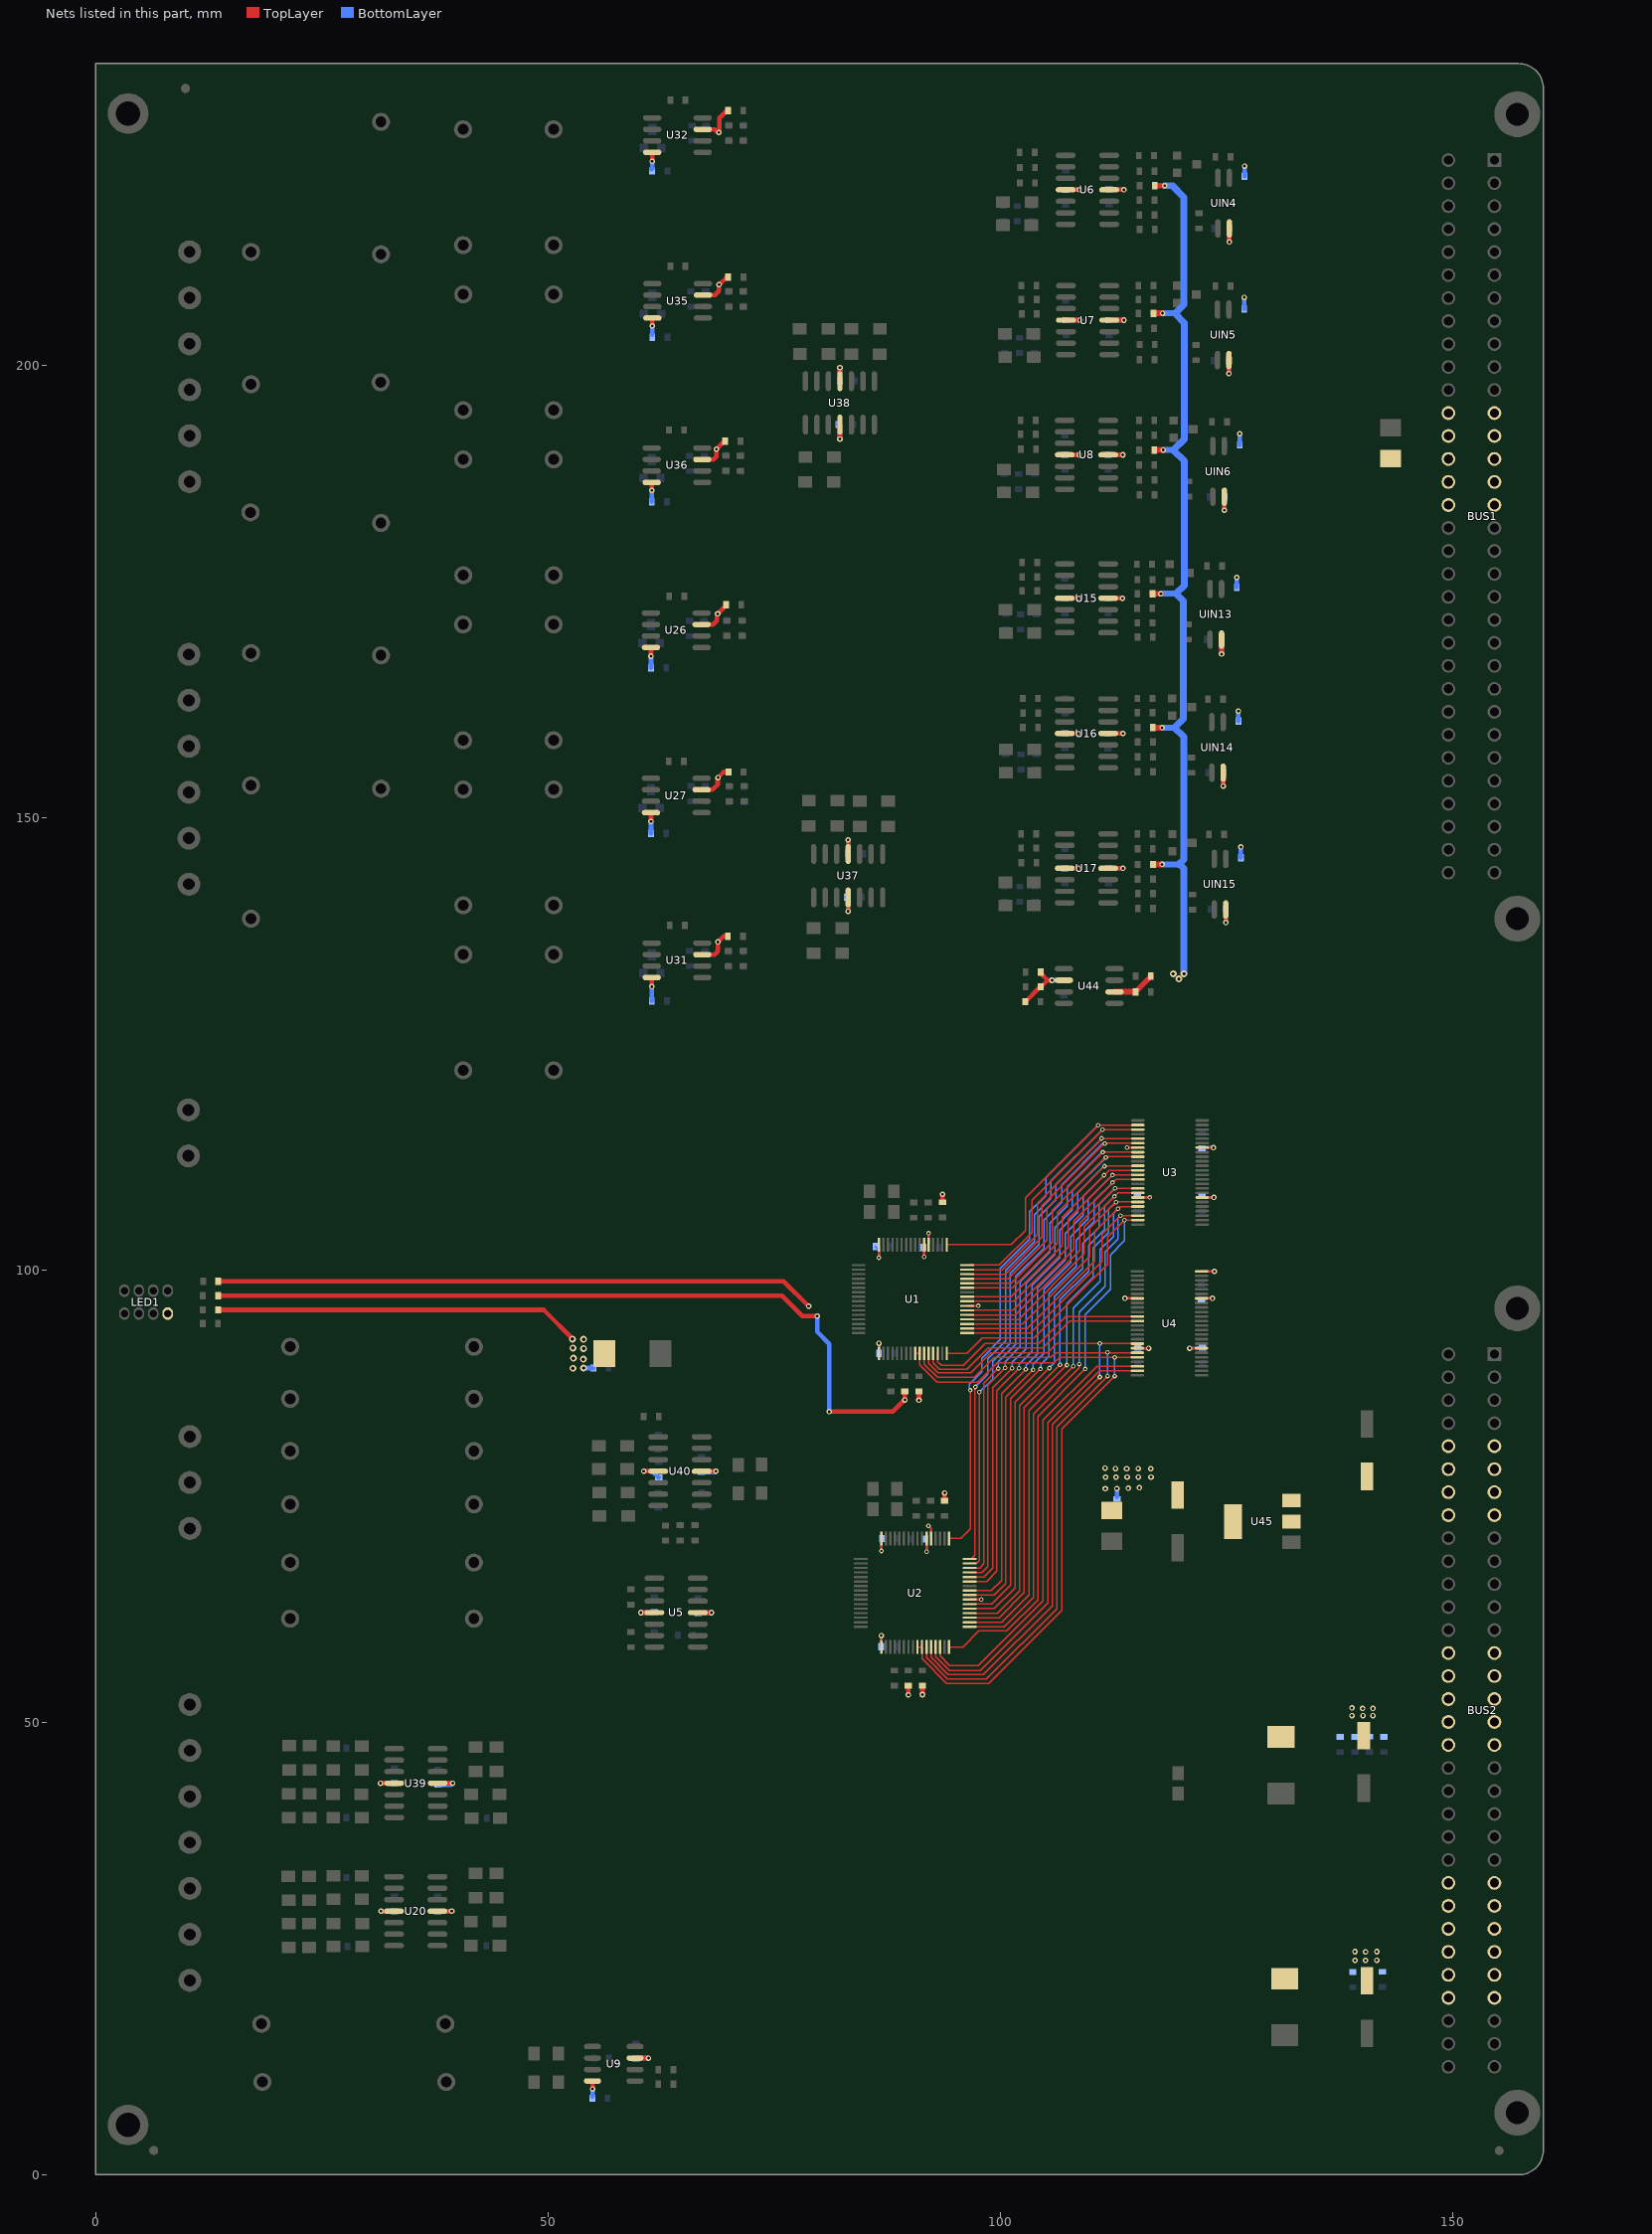
[diagram p0: the nets of this part, all layers, seen from the top]
# Altium PCB MISC80584.PCBDoc (part 3 of 7)
Units mm, origin at the board's own origin, x right, y up, seen from the top; angles counter-clockwise.
Board outline 160.02 x 233.3 mm, 4 copper layers (TopLayer, GND, POWER, BottomLayer); 386 components, 266 nets, 1374 pads, 640 vias.

## Part data
BUS1 BUS2: "Euro-style pin header, 64 positions"
C1 C2 C3 C7 C8 C18 C19 C22 C24 C25 C26 C119 C120 C121 C122 C123 C124 C128 C129 C156 C157 C158 C159 C163 C164 C165 C171 C173 C174 C175 C176 C177 C178 C179 C180 C181 C182 C183 C184 C192 C193 C194 C195 C196 C197 C204 C205 C206 C215 C216 C217 C218 C219 C220 C224 C230 C231 C232 C233 C234 C235 C238 C239 C240 C249 C251 C252 C253 C254 C255 C256 C257 C261 C262: library part CAP, "Capacitor"
C4 C5 C6 C9 C10 C11 C12 C13 C14 C15 C16 C17 C20 C21 C23 C27 C82 C83 C84 C85 C88 C89 C92 C93 C96 C97 C100 C101 C104 C113 C118 C125 C126 C130 C132 C135 C136 C139 C142 C143 C146 C147 C148 C149: library part CAP
CT1 CT2 CT3 CT17: library part EC
CT4 CT7 CT8 CT13 CT16: library part "CAPACITOR POL", "Capacitor"
D1 D2 D8 D9 D10 D11 D12 D13 D14 D15 D16 D17 D18 D20 D21 D22 D24 D25 D26 D27 D28 D29 D30 D31 D32 D33 D60 D61 D62 D63 D64 D65 D80 D81 D83 D84 D85 D89 D90 D91 D94 D95 D96 D97: library part DIODE-S
D42 D44 D46 D48 D51 D53: library part DDIODEB
J1 J2: "Connector"
L1: library part INDUCTOR
Q8 Q9 Q10 Q17 Q23 Q24: library part NPN, "NPN Transistor"
R1 R2 R3 R4 R5 R6 R7 R8 R9 R10 R11 R12 R13 R14 R23 R24 R25 R26 R27 R28 R29 R30 R31 R32 R33 R34 R35 R36 R37 R38 R40 R48 R57 R58 R59 R67 R70 R71 R76 R85 R86 R87 R93 R97 R100 R105 R106 R108 R110 R111 R113 R117 R118 R119 R120 R124 R125 R126 R130 R131 R132 R133 R137 R138 R139 R145 R146 R147 R150 R151 R152 R155 R156 R157 R161 R162 R165 R168 R171 R174 R211 R224 R225 R339 R340 R341 R342 R349 R350 R351 R353 R354 R355 R357 R358 R359 R360 R361 R362 R364 R365 R366 R372 R373 R374 R375 R376 R377 R379 R380 R381 R382 R383 R384 R399 R400 R401 R414 R423 R430 R431 R435 R437 R438 R444 R445 R446 R450 R451 R452 R459 R460 R461 R486 R487 R488 R491 R492 R493 R503 R506 R507 R510 R511 R512 R591 R592 R593 R600 R601 R602 R605 R607 R608 R609 R611 R612: library part RES2
SPT1 SPT2 SPT3 SPT4 SPT5 SPT6: library part SPT
U3 U4: library part SN74LVCH16T245, "TI SN74LVCH16T245DGGR"
U5 U20 U37 U38 U39 U40: "Low Power Quad Operational Amplifier"
U6 U7 U8 U15 U16 U17: library part TL084
U26 U27 U31 U32 U35 U36: library part LM101
U44: "U?"
U45: library part 7810
UIN4 UIN5 UIN6 UIN13 UIN14 UIN15: library part 521-1, "Optoisolator"

## Free pads (board coordinates)
  round 1 smd mask+1.5: 0(6.426,2.718) 0(9.931,230.581) 0(155.143,2.692)
  round 1 smd far side mask+1.5: 0(6.426,2.718) 0(9.931,230.581) 0(155.143,2.692)
  round 4.5 hole 2.7: 1(3.592,5.524) 1(3.592,227.823)

## Via types
v1: diameter 0.61, hole 0.305, TopLayer to BottomLayer, 342 vias
v2: diameter 0.762, hole 0.381, TopLayer to BottomLayer, 197 vias
v3: diameter 0.508, hole 0.254, TopLayer to BottomLayer, 101 vias

## Nets (pads, with @x,y where several pads share a name; then routed paths per layer and width w, separated by ;. In a path a pad name is that pad's centre, name@x,y a point inside that pad or via, vN(x,y) a via of type N, cw(c..) or ccw(c..) an arc to the next point about the centre after c; other vN are vias at no path point)
+3.3V: C1.2 C3.1 C8.1 CT16.1 CT17.1 R33.2 R34.2 R342.2 R605.2 R607.2 R609.2 R611.2 U1.23 U2.23 U3.7 U3.18 U4.24 U4.31 U4.42 U45.2 | length 105.4
  TopLayer w0.254: U1.23@96.339,96.055 v3(97.579,96.055) ; U2.23@96.593,63.594 v3(97.884,63.594)
  TopLayer w0.279: v1(113.764,96.873) U4.31@115.15,96.873 ; v3(113.979,113.529) U3.7@115.214,113.529 ; U4.42@115.15,91.373 v1(116.392,91.373) ; U3.18@115.214,108.029 v3(116.507,108.029) ; U4.24@122.25,99.873 v1(123.673,99.873)
  TopLayer w0.508: R342.2@13.538,97.18 75.87,97.18 78.13,94.92 v1(79.756,94.92) ; v1(81.102,84.353) 88.113,84.353 v1@89.408,85.649 ; v1(89.459,85.649) R607.2@89.459,86.589 ; v1(89.84,53.061) R611.2@89.84,54.077 ; v1(91.008,85.623) R605.2@91.008,86.589 ; v1(91.389,53.086) R609.2@91.389,54.077 ; R33.2@93.624,107.493 v1(93.624,108.382) ; R34.2@93.853,74.524 v1(93.853,75.387)
  BottomLayer w0.254: v3(97.579,96.055) v3@97.612,96.088 ; v3(97.884,63.594) v3@97.892,63.602
  BottomLayer w0.279: v1@113.741,96.85 v1(113.764,96.873) ; C8.1@115.138,108.052 116.357,108.052 v3@116.408,108.001 ; C1.2@115.189,91.364 v1@116.256,91.364 ; v1(116.392,91.373) v1@116.484,91.465 ; v3(116.507,108.029) v3@116.51,108.026
  BottomLayer w0.508: v1(79.756,94.92) 79.756,93.193 81.102,91.846 v1(81.102,84.353) ; v1@89.433,85.623 v1(89.459,85.649) ; v1@112.878,75.819 112.878,74.981 C3.1@112.903,74.955
  other v1: 111.608,75.844 112.878,75.87 114.148,75.895 115.367,75.946 111.633,77.114 112.776,77.114 114.021,77.14 115.265,77.14 116.662,77.14 113.97,78.054 116.637,78.054 112.725,78.08 115.24,78.08 111.582,78.13
+5V: BUS1.A12 BUS1.A13 BUS1.A14 BUS1.A15 BUS1.A16 BUS1.C12 BUS1.C13 BUS1.C14 BUS1.C15 BUS1.C16 BUS2.A5 BUS2.A6 BUS2.A7 BUS2.A8 BUS2.C5 BUS2.C6 BUS2.C7 BUS2.C8 C2.1 C7.2 C18.1 C24.1 C119.1 C120.1 C128.1 C129.1 C156.2 C157.1 C158.1 C159.2 C163.1 C164.1 C165.2 C171.1 CT1.1 CT8.1 R339.2 U1.1 U1.37 U1.38 U1.48 U2.1 U2.37 U2.38 U2.48 U3.31 U3.42 U4.7 U4.18 U45.3 UIN4.4 UIN5.4 UIN6.4 UIN13.4 UIN14.4 UIN15.4 | length 111.3
  TopLayer w0.254: v3(86.589,101.371) U1.48@86.589,102.805 ; U2.1@86.843,58.344 v1(86.843,59.614) ; v3(86.843,68.961) U2.48@86.843,70.344 ; v3(91.589,101.444) U1.38@91.589,102.805 ; v3(91.843,68.889) U2.38@91.843,70.344 ; v3(92.05,71.73) 92.343,71.437 U2.37@92.343,70.344 ; v3(92.061,104.076) 92.089,104.076 U1.37@92.089,102.805
  TopLayer w0.279: U1.1@86.589,90.805 v1@86.589,91.948 ; v1(120.938,91.373) U4.7@122.25,91.373 ; U4.18@122.25,96.873 v1(123.441,96.873) ; U3.31@122.314,108.029 v1(123.619,108.029) ; U3.42@122.314,113.529 v1(123.562,113.529)
  TopLayer w0.508: R339.2@13.564,98.755 76.048,98.755 78.816,95.987 v1(78.816,96.012) ; v1(124.46,168.072) UIN13.4@124.46,169.672 ; v1(124.638,153.492) UIN14.4@124.638,154.965 ; v1(124.765,183.972) UIN6.4@124.765,185.471 ; v1(124.917,138.405) UIN15.4@124.917,139.852 ; v1(125.273,199.085) UIN5.4@125.273,200.558 ; v1(125.324,213.614) UIN4.4@125.324,215.113
  BottomLayer w0.254: C119.1@86.208,102.591 86.589,102.21 v3@86.589,101.448 ; C129.1@86.843,58.369 v1@86.843,59.436 ; v3@86.843,69.139 C24.1@86.843,70.333 ; C18.1@91.491,102.489 91.592,102.387 v3@91.592,101.524 ; v3@91.846,69.012 C120.1@91.846,70.358
  BottomLayer w0.279: C128.1@86.589,90.78 v1@86.589,91.821 ; v1@121.031,91.389 C2.1@122.326,91.389 ; C171.1@122.25,96.876 v1@123.317,96.876 ; C165.2@122.276,113.589 v1@123.52,113.589 ; C7.2@122.482,108.029 v1(123.619,108.029) ; v1(123.441,96.873) v1@123.444,96.876 ; v1(123.562,113.529) v1@123.571,113.538
  BottomLayer w0.508: v1(124.46,168.072) C159.2@124.46,169.469 ; v1(124.638,153.492) C163.1@124.638,154.813 ; v1(124.765,183.972) C158.1@124.765,185.268 ; C164.1@124.892,139.878 124.917,139.852 v1(124.917,138.405) ; v1(125.273,199.085) C157.1@125.273,200.457 ; v1(125.324,213.614) 125.324,214.96 C156.2@125.349,214.986
  other v1: 86.589,91.923
+5VREF: C148.1 C149.2 R155.2 R156.2 R157.2 R379.2 R380.2 R381.2 U44.6 | length 110.3
  TopLayer w0.635: U44.6@112.624,130.759 114.859,130.759 114.91,130.708 116.611,132.41 C149.2@116.611,132.486 ; R379.2@116.815,174.727 v1(117.754,174.727) ; R380.2@116.84,159.944 v1(117.881,159.944) ; R381.2@116.865,144.831 v1(117.881,144.831) ; R156.2@116.942,205.74 v1(117.932,205.74) ; R157.2@117.018,190.627 v1(118.008,190.627) ; R155.2@117.069,219.837 v1(118.161,219.837)
  BottomLayer w0.635: v1@117.78,174.752 119.405,174.752 ; v1@117.932,159.944 119.253,159.944 ; v1@117.983,144.831 119.71,144.831 ; v1@118.008,205.74 119.278,205.74 ; v1@118.034,190.627 119.151,190.627
  BottomLayer w0.762: v1(118.161,219.837) 119.024,219.837 120.294,218.567 120.294,206.705 119.329,205.74 119.278,205.74 120.345,204.673 120.345,191.821 119.151,190.627 119.126,190.602 119.151,190.602 120.345,189.408 120.345,175.666 119.431,174.752 120.218,173.965 120.218,160.909 119.253,159.944 120.269,158.928 120.269,145.39 119.71,144.831 119.837,144.831 120.269,144.399 v2@120.269,132.817
  other v2: 119.736,132.182 119.126,132.74 120.294,132.74
+15V: BUS2.A14 BUS2.A15 BUS2.A16 BUS2.A17 BUS2.A18 BUS2.C14 BUS2.C15 BUS2.C16 BUS2.C17 BUS2.C18 C146.1 C147.1 C173.2 C174.1 C175.1 C176.2 C177.1 C178.2 C179.2 C180.1 C181.1 C182.2 C183.2 C184.1 C215.1 C216.2 C217.2 C218.1 C219.2 C220.2 C224.1 C230.2 C231.1 C232.1 C233.2 C234.1 C235.2 CT2.1 CT4.1 CT7.1 R224.2 R340.2 R486.1 R487.1 R488.1 R503.1 R506.1 R507.1 U5.4 U6.4 U7.4 U8.4 U9.7 U15.4 U16.4 U17.4 U20.4 U26.7 U27.7 U31.7 U32.7 U35.7 U36.7 U37.4 U38.4 U39.4 U40.4 U44.2 | length 117.5
  TopLayer w0.508: R340.2@13.538,95.606 49.53,95.606 v2@52.73,92.405 ; v1(31.496,43.307) U39.4@33.008,43.307 ; v1(31.547,29.159) U20.4@32.982,29.159 ; U9.7@59.627,12.929 v1(61.112,12.929) ; v1(60.274,62.154) U5.4@61.76,62.154 ; v1(60.579,77.775) U40.4@62.192,77.775 ; U27.7@66.98,153.086 68.199,153.086 68.758,153.645 v1@68.758,154.381 ; U26.7@66.98,171.348 68.25,171.348 68.682,171.78 v1@68.682,172.441 ; U31.7@67.056,134.874 68.428,134.874 68.783,135.23 v1@68.783,136.246 ; U36.7@67.056,189.586 68.301,189.586 68.605,189.89 68.605,190.729 v1(68.631,190.729) C181.1@69.596,191.694 ; U32.7@67.107,226.06 68.453,226.06 v1@68.783,225.73 ; U35.7@67.132,207.747 68.478,207.747 68.91,208.178 v1@68.91,208.864 ; v1(68.758,172.517) v1@68.682,172.441 ; v1(68.783,136.271) v1@68.783,136.246 ; v1@68.796,225.742 v1@68.809,225.73 ; v1(68.809,154.432) v1@68.758,154.381 ; v1@68.809,225.704 v1@68.809,225.73 ; v1@68.834,225.704 v1@68.809,225.73 ; v1@68.834,225.781 v1@68.885,225.831 ; v1(68.885,225.704) v1@68.885,225.831 ; v1(68.91,208.915) v1@68.91,208.864 ; C180.1@69.672,173.431 v1@68.682,172.441 ; C184.1@69.748,209.702 v1@68.91,208.864 ; C183.2@69.774,228.143 68.961,227.33 68.961,225.908 v1@68.885,225.831 ; C178.2@69.85,136.881 69.418,136.881 v1@68.783,136.246 ; C179.2@69.952,155.042 69.418,155.042 v1@68.758,154.381 ; U38.4@82.271,198.234 v1(82.271,199.72) ; U37.4@83.185,145.986 v1(83.185,147.549) ; R224.2@102.768,129.667 C147.1@104.318,131.216 ; C147.1@104.572,131.369 105.232,132.029 ; C146.1@104.623,132.639 105.232,132.029 ; v1(105.715,132.029) 105.232,132.029 ; U17.4@107.125,144.399 v1(108.61,144.399) ; U16.4@107.125,159.309 v1(108.61,159.309) ; U15.4@107.125,174.244 v1(108.661,174.244) ; U8.4@107.125,190.094 v1(108.737,190.094) ; U6.4@107.226,219.38 v1(108.737,219.38) ; U7.4@107.252,204.978 v1(108.814,204.978)
  BottomLayer w0.508: v1(31.496,43.307) C235.2@32.817,43.307 ; v1@31.623,29.185 31.674,29.134 C230.2@33.045,29.134 ; v2@54.178,89.205 54.204,89.179 C182.2@55.016,89.179 ; C220.2@59.792,12.903 59.817,12.929 v1(61.112,12.929) ; v1(60.274,62.154) C177.1@61.62,62.154 ; v1@60.63,77.775 61.544,77.775 C234.1@62.23,77.089 ; v1(68.783,136.271) v1@68.809,136.296 ; C224.1@82.194,198.247 82.271,198.323 v1(82.271,199.72) ; C233.2@83.185,146.228 v1(83.185,147.549) ; v1(105.715,132.029) C216.2@106.909,132.029 ; C217.2@107.239,159.334 107.264,159.309 v1(108.61,159.309) ; C218.1@107.239,174.269 107.264,174.244 v1(108.661,174.244) ; C231.1@107.29,144.399 v1(108.61,144.399) ; C232.1@107.29,190.094 v1(108.737,190.094) ; C215.1@107.34,219.405 107.366,219.38 v1(108.737,219.38) ; C219.2@107.467,204.978 v1(108.814,204.978) ; R503.1@126.136,175.438 v1(126.136,176.555) ; R506.1@126.314,160.655 v1(126.314,161.773) ; R488.1@126.467,191.186 v1(126.467,192.43) ; R507.1@126.594,145.567 v1(126.594,146.761) ; R487.1@126.949,206.223 v1(126.949,207.493) ; R486.1@127,220.878 v1(127,221.996)
  other v1: 138.862,50.775 140.081,50.775 141.199,50.775 140.056,51.562 141.199,51.562 138.862,51.613
  other v2: 52.756,89.154 53.95,89.179 53.924,90.145 52.807,90.272 53.95,91.338 52.756,91.389 53.95,92.354 52.705,92.38
-15V: BUS2.A24 BUS2.A25 BUS2.A26 BUS2.A27 BUS2.A28 BUS2.A29 BUS2.C24 BUS2.C25 BUS2.C26 BUS2.C27 BUS2.C28 BUS2.C29 C192.2 C193.1 C194.2 C195.1 C196.1 C197.2 C204.2 C205.2 C206.1 C238.2 C239.1 C240.1 C249.1 C251.2 C252.1 C253.2 C254.1 C255.1 C256.2 C257.2 C261.2 C262.1 CT3.2 CT13.2 LED1.8 U5.11 U6.11 U7.11 U8.11 U9.4 U15.11 U16.11 U17.11 U20.11 U26.4 U27.4 U31.4 U32.4 U35.4 U36.4 U37.11 U38.11 U39.11 U40.11 | length 52.4
  TopLayer w0.508: U20.11@37.782,29.159 v1(39.37,29.159) ; U39.11@37.808,43.307 v1(39.472,43.307) ; v1(54.927,9.513) U9.4@54.927,10.389 ; v1(61.392,149.581) U27.4@61.392,150.546 ; v1(61.392,167.843) U26.4@61.392,168.808 ; v1(61.468,131.318) U31.4@61.468,132.334 ; v1(61.468,186.157) U36.4@61.468,187.046 ; v1(61.519,222.529) U32.4@61.519,223.52 ; v1(61.544,204.343) U35.4@61.544,205.207 ; U5.11@66.56,62.154 v1(68.072,62.154) ; U40.11@66.992,77.775 v1(68.555,77.775) ; v1(82.271,191.846) U38.11@82.271,193.434 ; v1(83.185,139.649) U37.11@83.185,141.186 ; U17.11@111.925,144.399 v1(113.563,144.399) ; U16.11@111.925,159.309 v1(113.563,159.309) ; U15.11@111.925,174.244 v1(113.513,174.244) ; U8.11@111.925,190.094 v1(113.538,190.094) ; U6.11@112.026,219.38 v1(113.665,219.38) ; U7.11@112.052,204.978 v1(113.665,204.978)
  BottomLayer w0.508: C194.2@37.846,43.129 39.243,43.129 v1@39.421,43.307 ; C192.2@37.922,29.185 37.948,29.159 v1(39.37,29.159) ; C195.1@54.915,8.687 54.927,8.699 v1(54.927,9.513) ; C254.1@61.392,148.26 v1@61.392,149.504 ; C252.1@61.392,166.548 61.392,167.742 v1@61.417,167.767 ; v1@61.443,186.131 61.468,186.106 C249.1@61.468,184.887 ; C261.2@61.443,221.64 61.519,221.717 v1(61.519,222.529) ; C253.2@61.468,129.743 v1@61.468,131.242 ; C251.2@61.519,203.352 61.544,203.378 v1(61.544,204.343) ; C196.1@66.751,62.103 66.777,62.128 68.097,62.128 v1(68.072,62.154) ; C197.2@66.98,77.673 68.453,77.673 v1(68.555,77.775) v1@68.58,77.8 ; C240.1@82.042,193.523 82.271,193.294 v1(82.271,191.846) ; C262.1@82.956,141.224 83.185,140.995 v1(83.185,139.649) ; C256.2@111.938,174.244 v1@113.462,174.244 ; C257.2@112.014,219.38 v1@113.64,219.38 ; C238.2@112.039,159.283 113.538,159.283 v1(113.563,159.309) ; C239.1@112.065,190.068 113.513,190.068 v1(113.538,190.094) ; C255.1@112.141,144.399 v1(113.563,144.399) ; C193.1@112.268,205.003 112.293,204.978 v1(113.665,204.978) ; v1@113.487,174.219 v1(113.513,174.244)
  other v1: 139.217,23.724 140.36,23.724 141.605,23.749 140.386,24.663 139.192,24.689 141.605,24.689
AD_BUSY1: U1.14 U4.35 | length 25.4
  TopLayer w0.152: U1.14@93.089,90.805 93.089,89.893 93.497,89.484 95.91,89.484 98.349,91.923 104.292,91.923 107.243,94.873 U4.35@115.15,94.873
AD_BUSY2: U2.14 U4.46 | length 48.6
  TopLayer w0.152: U2.14@93.343,58.344 93.343,57.381 94.412,56.312 97.587,56.312 104.724,63.449 104.724,83.414 110.683,89.373 U4.46@115.15,89.373
AD_CON: U1.9 U1.10 U2.9 U2.10 U4.44 | length 79.8
  TopLayer w0.152: U1.9@90.602,90.805 U1.10@91.089,90.805 91.089,89.556 93.015,87.63 97.536,87.63 99.644,89.738 105.918,89.738 106.553,90.373 U4.44@115.15,90.373 ; U2.9@90.881,58.344 U2.10@91.343,58.344 91.343,57.07 94.082,54.331 98.73,54.331 106.782,62.382 106.782,82.423 v3(112.649,88.29)
  BottomLayer w0.152: v3(112.649,88.29) v3(112.649,90.373)
AD_CS1: U1.13 U4.36 | length 26.1
  TopLayer w0.152: U1.13@92.589,90.805 92.589,89.733 93.269,89.052 96.317,89.052 98.679,91.415 104.724,91.415 107.682,94.373 U4.36@115.15,94.373
AD_CS2: U2.13 U4.47 | length 49.4
  TopLayer w0.152: U2.13@92.843,58.344 92.843,57.297 94.412,55.728 97.765,55.728 105.258,63.221 105.258,83.16 110.971,88.873 U4.47@115.15,88.873
AD_D0: U1.16 U2.16 U3.23 | length 86.9
  TopLayer w0.152: U1.16@94.089,90.805 96.291,90.805 97.993,92.507 103.734,92.507 111.836,100.609 111.836,103.632 v3@113.733,105.529 ; U2.16@94.343,58.344 95.86,58.344 97.638,60.122 100.686,60.122 104.14,63.576 104.14,83.845 v3(109.372,89.078) ; v3(113.724,105.529) v3@113.733,105.529 ; U3.23@115.164,105.529 v3@113.733,105.529
  BottomLayer w0.152: v3(109.372,89.078) 109.372,95.072 112.192,97.892 112.192,101.702 113.741,103.251 v3@113.741,105.588
AD_D1: U1.17 U2.17 U3.22 | length 80.5
  TopLayer w0.152: U1.17@96.339,93.055 103.342,93.055 111.252,100.965 111.252,103.988 v3(113.284,106.02) 113.293,106.029 U3.22@115.164,106.029 ; U2.17@96.593,60.594 100.421,60.594 103.657,63.83 103.657,84.125 108.712,89.179 v3@108.712,89.586
  BottomLayer w0.152: v3(108.712,89.611) 108.712,95.352 111.582,98.222 111.582,101.981 113.03,103.429 113.03,105.766 v3(113.284,106.02)
AD_D2: U1.18 U2.18 U3.20 | length 81.2
  TopLayer w0.152: U1.18@96.339,93.555 102.953,93.555 110.414,101.016 110.414,104.242 113.201,107.029 ; U2.18@96.593,61.094 100.159,61.094 103.149,64.084 103.149,84.455 v3(108.077,89.383) ; v3(113.005,106.782) 113.005,106.82 113.201,107.017 113.201,107.029 ; U3.20@115.164,107.029 113.201,107.029
  BottomLayer w0.152: v3(108.077,89.383) 108.077,95.783 111.049,98.755 111.049,102.26 112.497,103.708 112.497,106.274 v3@113.017,106.794
AD_D3: U1.19 U2.19 U3.19 | length 80.7
  TopLayer w0.152: U1.19@96.339,94.055 102.437,94.055 109.88,101.498 109.88,104.623 v3@112.787,107.529 ; U2.19@96.593,61.594 99.872,61.594 102.641,64.364 102.641,84.785 v3(107.366,89.51) ; v3(112.787,107.504) v3@112.787,107.529 ; U3.19@115.164,107.529 v3@112.787,107.529
  BottomLayer w0.152: v3(107.366,89.51) 107.366,96.317 110.261,99.212 110.261,102.438 111.989,104.165 111.989,106.731 v3@112.725,107.467
AD_D4: U1.20 U2.20 U3.17 | length 80.8
  TopLayer w0.152: U1.20@96.339,94.555 101.997,94.555 109.296,101.854 109.296,104.8 v3@112.636,108.14 ; U2.20@96.593,62.094 99.66,62.094 102.108,64.541 102.108,85.039 v3(106.604,89.535) ; v3(112.611,108.14) v3@112.636,108.14 ; U3.17@115.164,108.529 113.025,108.529 v3@112.636,108.14
  BottomLayer w0.152: v3(106.604,89.535) 106.604,96.723 109.753,99.873 109.753,102.718 111.531,104.496 111.531,107.061 v3(112.611,108.14)
AD_D5: U1.21 U2.21 U3.16 | length 81.1
  TopLayer w0.152: U1.21@96.339,95.055 101.659,95.055 108.763,102.159 108.763,105.181 112.61,109.029 v3(112.687,109.029) 113.081,109.029 U3.16@115.164,109.029 ; U2.21@96.593,62.594 99.348,62.594 101.625,64.872 101.625,85.395 v3(105.41,89.179)
  BottomLayer w0.152: v3(105.41,89.179) 105.994,89.764 105.994,97.079 109.118,100.203 109.118,102.921 110.922,104.724 110.922,107.29 v3@112.674,109.042
AD_D6: U1.22 U2.22 U3.14 | length 81.2
  TopLayer w0.152: U1.22@96.339,95.555 101.422,95.555 108.128,102.26 108.128,105.385 112.243,109.499 112.772,110.029 U3.14@115.164,110.029 ; U2.22@96.593,63.094 99.035,63.094 101.143,65.202 101.143,85.776 v3(104.445,89.078)
  BottomLayer w0.152: v3(104.445,89.078) 104.496,89.129 104.496,89.586 105.385,90.475 105.385,97.409 108.382,100.406 108.382,103.327 110.388,105.334 110.388,107.645 112.395,109.652 v3(112.395,109.677)
AD_D7: U1.24 U2.24 U3.13 | length 81
  TopLayer w0.152: U1.24@96.339,96.555 101.533,96.555 107.518,102.54 107.518,105.639 v3@112.409,110.529 ; U2.24@96.593,64.094 99.324,64.094 100.609,65.38 100.609,85.979 v3(103.632,89.002) ; v3(112.409,110.502) v3@112.409,110.529 ; U3.13@115.164,110.529 v3@112.409,110.529
  BottomLayer w0.152: v3(103.632,89.002) 103.632,89.611 104.826,90.805 104.826,97.892 107.772,100.838 107.772,103.734 109.728,105.689 109.728,107.823 v3@112.37,110.465
AD_D8: U1.25 U2.25 U3.12 | length 79.9
  TopLayer w0.152: U1.25@96.339,97.055 101.17,97.055 106.858,102.743 106.858,105.867 111.417,110.426 v3(111.481,110.49) 112.02,111.029 U3.12@115.164,111.029 ; U2.25@96.593,64.594 99.011,64.594 100.127,65.71 100.127,86.36 v3(102.819,89.052)
  BottomLayer w0.152: v3(102.819,89.052) 102.819,89.484 104.089,90.754 104.089,98.069 107.163,101.143 107.163,104.064 109.144,106.045 109.144,108.153 v3(111.481,110.49)
AD_D9: U1.27 U2.27 U3.11 | length 80.4
  TopLayer w0.152: U1.27@96.339,98.055 101.382,98.055 106.299,102.972 106.299,106.324 v3@111.504,111.529 ; U2.27@96.593,65.594 98.487,65.594 99.619,66.726 99.619,85.7 ; 99.619,86.589 99.619,85.7 ; v3(102.083,89.154) 99.619,86.69 99.619,85.7 ; v3(111.504,111.483) v3@111.504,111.529 ; U3.11@115.164,111.529 v3@111.504,111.529
  BottomLayer w0.152: v3(102.083,89.154) 102.083,89.586 103.505,91.008 103.505,98.298 106.604,101.397 106.604,104.445 108.534,106.375 108.534,108.56 v3@111.404,111.43
AD_D10: U1.28 U2.28 U3.9 | length 80.6
  TopLayer w0.152: U1.28@96.339,98.555 101.197,98.555 105.74,103.099 105.74,106.604 v3@111.665,112.529 ; U2.28@96.593,66.094 98.199,66.094 99.162,67.056 99.162,86.284 ; 99.162,86.614 99.162,86.284 ; v3(101.295,89.154) 99.162,87.02 99.162,86.284 ; v3(111.665,112.453) v3@111.665,112.529 ; U3.9@115.164,112.529 v3@111.665,112.529
  BottomLayer w0.152: v3(101.295,89.154) 101.295,89.789 102.819,91.313 102.819,98.527 106.045,101.752 106.045,104.724 107.975,106.655 107.975,108.763 v3(111.665,112.453)
AD_D11: U1.29 U2.29 U3.8 | length 80.6
  TopLayer w0.152: U1.29@96.339,99.055 100.884,99.055 105.156,103.327 105.156,106.832 v3@111.353,113.029 ; U2.29@96.593,66.594 97.963,66.594 98.628,67.259 98.628,85.903 ; 98.628,86.487 98.628,85.903 ; v3(100.533,89.205) 98.628,87.3 98.628,85.903 ; v3(111.329,113.029) v3@111.353,113.029 ; U3.8@115.164,113.029 v3@111.353,113.029
  BottomLayer w0.152: v3(100.533,89.205) 100.533,89.891 102.21,91.567 102.21,98.73 105.461,101.981 105.461,105.181 107.391,107.112 107.391,109.195 v3@111.227,113.03
AD_D12: U1.30 U2.30 U3.6 | length 80.7
  TopLayer w0.152: U1.30@96.339,99.555 100.546,99.555 104.623,103.632 104.623,107.137 v3@111.514,114.029 ; U2.30@96.593,67.094 97.726,67.094 98.171,67.539 98.171,87.528 v3(99.771,89.129) ; v3@111.557,114.029 U3.6@115.164,114.029
  BottomLayer w0.152: v3(99.771,89.129) 99.771,89.84 101.702,91.77 101.702,99.314 104.8,102.413 104.8,105.512 106.782,107.493 106.782,109.449 111.303,113.97 v3@111.531,113.97
  other v3: 111.557,113.987
AD_D13: U1.31 U2.31 U3.5 | length 80.4
  TopLayer w0.152: U1.31@96.339,100.055 100.207,100.055 104.089,103.937 104.089,107.391 v3@111.227,114.529 ; U2.31@96.593,67.594 97.388,67.594 97.688,67.894 v3(97.688,86.512) ; v3(111.201,114.554) v3@111.227,114.529 ; U3.5@115.164,114.529 v3@111.227,114.529
  BottomLayer w0.152: v3(97.688,86.512) 99.136,87.96 99.136,89.941 101.067,91.872 101.067,99.619 104.267,102.819 104.267,105.893 106.121,107.747 106.121,109.474 v3(111.201,114.554)
AD_D14: U1.32 U2.32 U3.3 | length 80.8
  TopLayer w0.152: U1.32@96.339,100.555 99.895,100.555 103.505,104.165 103.505,107.721 111.313,115.529 v3(111.318,115.529) U3.3@115.164,115.529 ; U2.32@96.593,68.094 96.796,68.094 97.206,68.504 97.206,87.071 v3(97.231,87.097)
  BottomLayer w0.152: v3(97.231,87.097) 98.603,88.468 98.603,90.17 100.609,92.177 100.609,99.974 103.784,103.149 103.784,106.147 105.588,107.95 105.588,109.855 v3@111.277,115.545
AD_D15: U1.33 U2.33 U3.2 | length 82
  TopLayer w0.152: U1.33@94.089,102.805 101.205,102.805 102.768,104.369 102.768,107.975 v3(110.82,116.027) 110.822,116.029 U3.2@115.164,116.029 ; U2.33@94.343,70.344 95.642,70.344 96.698,71.399 96.698,86.665 v3@96.723,86.69 ; U3.2@115.087,116.027 U3.2@115.113,116.002
  BottomLayer w0.152: v3(96.672,86.716) 96.596,86.792 96.596,87.401 97.942,88.748 97.942,90.272 100,92.329 100,100.178 103.251,103.429 103.251,106.451 105.029,108.229 105.029,110.236 v3(110.82,116.027)
AD_RD: U1.12 U2.12 U4.41 | length 75.6
  TopLayer w0.152: U1.12@92.089,90.805 92.089,89.674 93.116,88.646 96.749,88.646 98.958,90.856 105.232,90.856 106.249,91.873 U4.41@115.15,91.873 ; U2.12@92.343,58.344 92.343,57.213 94.234,55.321 98.146,55.321 105.74,62.916 105.74,82.931 v3(110.998,88.189)
  BottomLayer w0.152: v3(110.998,88.189) v3(110.998,91.897)
AD_RST: U1.11 U2.11 U4.43 | length 77
  TopLayer w0.152: U1.11@91.589,90.805 91.589,89.59 93.04,88.138 97.104,88.138 99.314,90.348 105.613,90.348 106.138,90.873 U4.43@115.15,90.873 ; U2.11@91.843,58.344 91.843,57.154 94.183,54.813 98.476,54.813 106.248,62.586 106.248,82.017 106.223,82.042 106.223,82.652 v3(111.862,88.29)
  BottomLayer w0.152: v3(111.862,88.29) v3(111.862,90.907)